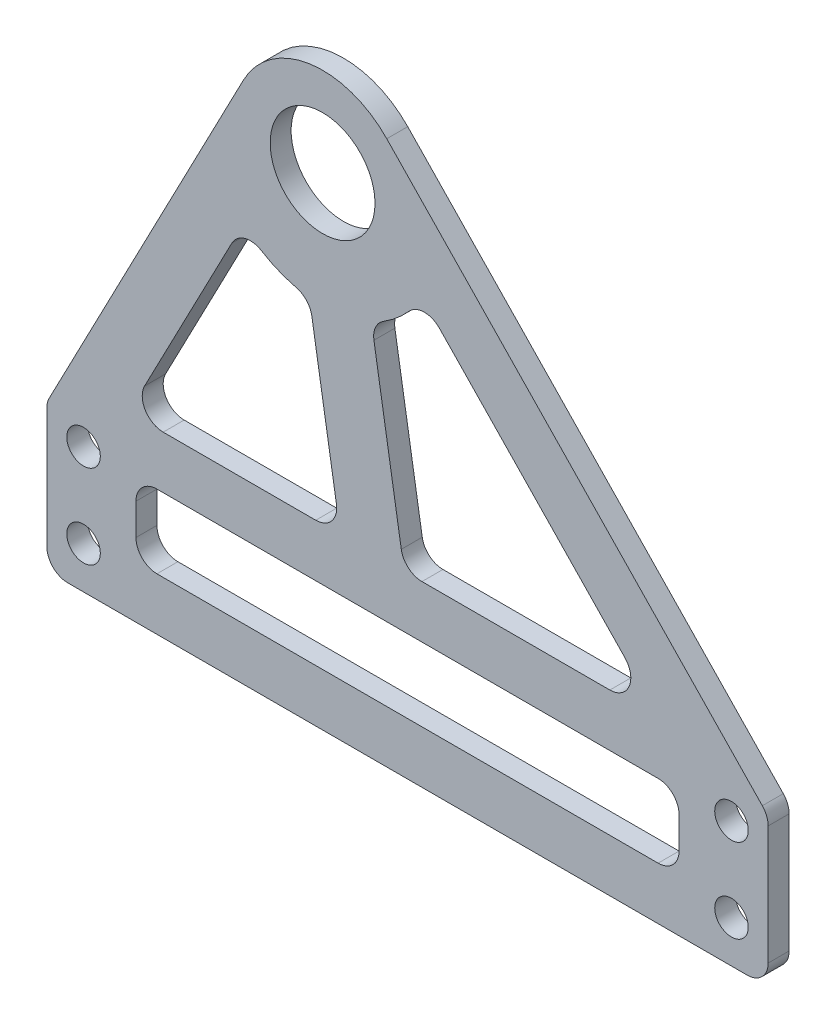
SolidWorks part; units mm, degrees
material "Thornel Mat VMA"
ref_plane "前视基准面" through (0, 0, 0) normal (0, 0, 1) x (1, 0, 0)
ref_plane "上视基准面" through (0, 0, 0) normal (0, 1, 0) x (1, 0, 0)
ref_plane "右视基准面" through (0, 0, 0) normal (1, 0, 0) x (0, 0, -1)
other "Configuration Table"
sketch "草图1" plane through (0, 0, 0) normal (0, 0, 1) x (1, 0, 0)
  line L0 (-26.8, 16.8667) -> (-26.8, -34) construction
  line L1 (43, 15.0741) -> (43, -34) construction
  line L2 (-26.8, -34) -> (43, -34) construction
  line L3 (-22.8, -34) -> (-22.8, -42) construction
  line L4 (8.1, -34) -> (8.1, 15.0741) construction
  line L5 (-26.3, -32.0608) -> (-26.3, -46)
  line L6 (-7.5372, 3.9294) -> (-26.3, -32.0608)
  line L7 (-26.3, -46) -> (42.5, -46)
  line L8 (42.5, -46) -> (42.5, -31.8677)
  line L9 (42.5, -31.8677) -> (6.1217, 5.897)
  circle A0 centre (0, 0) radius 5
  circle A1 centre (-22.8, -34) radius 1.6
  circle A2 centre (-22.8, -42) radius 1.6
  circle A3 centre (39, -42) radius 1.6
  circle A4 centre (39, -34) radius 1.6
  arc A5 (6.1217, 5.897) -> (-7.5372, 3.9294) centre (0, 0) ccw
  dimension "D3" = 10
  dimension "D5" = 3.2
  dimension "D6" = 3.2
  dimension "D10" = 17
  dimension "D1" = 26.8
  dimension "D2" = 43
  dimension "D4" = 34
  dimension "D7" = 8
  dimension "D8" = 4
  dimension "D9" = 0.5
  dimension "D11" = 4
  dimension "D12" = 0.5
  dimension "D13" = 4
  dimension "D14" = 4
extrude "凸台-拉伸1" add sketch "草图1" along normal blind 2
sketch "草图2" plane through (0, 0, 2) normal (0, 0, 1) x (1, 0, 0)
  line L0 (-22.8, -34) -> (-25.3, -34) construction
  line L1 (-25.3, -34) -> (-25.3, -18) construction
  line L2 (-25.3, -17.75) -> (15.7, -17.75) construction
  line L3 (-26.3, -32.0608) -> (-28.2703, -18.1713)
  line L4 (-6.0422, 5.9785) -> (-27.4325, -15.64)
  line L5 (-26.3, -32.0608) -> (-7.5372, 3.9294)
  circle A0 centre (-25.3, -18) radius 2.75 construction
  circle A1 centre (-25.3, -17.75) radius 2.5 construction
  circle A2 centre (-25.3, -17.75) radius 1.6
  circle A3 centre (15.7, -17.75) radius 1.6 construction
  arc A4 (-27.4325, -15.64) -> (-28.2703, -18.1713) centre (-25.3, -17.75) ccw
  arc A5 (6.1217, 5.897) -> (-7.5372, 3.9294) centre (0, 0) ccw construction
  arc A6 (-6.0422, 5.9785) -> (-7.5372, 3.9294) centre (0, 0) ccw
  dimension "D3" = 5.5
  dimension "D4" = 5
  dimension "D5" = 3.2
  dimension "D7" = 3.2
  dimension "D8" = 6
  dimension "D1" = 2.5
  dimension "D2" = 16
  dimension "D6" = 41
extrude "凸台-拉伸2" [suppressed] add sketch "草图2" against normal up to surface (3 mm away)
sketch "草图3" plane through (0, 0, 2) normal (0, 0, 1) x (1, 0, 0)
  circle A0 centre (15.7, -17.75) radius 1.6
  dimension "D1" = 3.2
extrude "切除-拉伸1" [suppressed] cut sketch "草图3" against normal up to surface (3 mm away)
sketch "草图4" [suppressed] plane through (0, 0, 3) normal (0, 0, 1) x (1, 0, 0)
  line L0 (0, 0) -> (-20.5, -17.75) construction
  line L1 (-20.5, -17.75) -> (-18, -34) construction
  line L2 (-18, -34) -> (39, -34) construction
  line L3 (39, -34) -> (20.5, -17.75) construction
  line L4 (20.5, -17.75) -> (0, 0) construction
  line L5 (0, 0) -> (10.5, -34) construction
  line L6 (-14.2121, -31) -> (-16.0014, -19.37)
  line L7 (-16.0014, -19.37) -> (-6.6873, -8.0951)
  line L8 (-14.2121, -31) -> (5.9104, -31)
  line L9 (5.9104, -31) -> (-0.4231, -10.4915)
  line L10 (13.2366, -31) -> (31.2197, -31)
  line L11 (31.2197, -31) -> (20.5364, -21.7498)
  line L12 (13.2366, -31) -> (6.6729, -9.7461)
  line L13 (16.5361, -18.2861) -> (6.6729, -9.7461)
  line L14 (-5.7822, 4.7766) -> (-22.8129, -15.8393) construction
  arc A2 (16.5361, -18.2861) -> (20.5364, -21.7498) centre (20.5, -17.75) ccw
  arc A3 (-6.6873, -8.0951) -> (-0.4231, -10.4915) centre (0, 0) ccw
  dimension "D1" = 10.5
  dimension "D8" = 8
  dimension "D2" = 7.5
  dimension "D3" = 4.2
  dimension "D4" = 3
  dimension "D5" = 3.5
  dimension "D6" = 3.5
  dimension "D7" = 3
extrude "切除-拉伸2" [suppressed] cut sketch "草图4" against normal through all
fillet "圆角1" [suppressed] radius 3
fillet "圆角2" [suppressed] radius 1
fillet "圆角3" [suppressed] radius 2
sketch "草图5" [suppressed] plane through (0, 0, 3) normal (0, 0, 1) x (1, 0, 0)
  line L0 (-18, -34) -> (-18, -42) construction
  line L1 (-13, -36) -> (34, -36)
  line L2 (-13, -36) -> (-13, -41.5)
  line L3 (-13, -41.5) -> (34, -41.5)
  line L4 (34, -36) -> (34, -41.5)
  line L5 (-18, -42) -> (39, -42) construction
  line L6 (-11.6384, -31) -> (1.8442, -31) construction
  dimension "D1" = 5
  dimension "D2" = 5
  dimension "D3" = 0.5
  dimension "D4" = 5
extrude "切除-拉伸3" [suppressed] cut sketch "草图5" against normal through all
fillet "圆角4" [suppressed] radius 2
sketch "草图6" plane through (0, 0, 2) normal (0, 0, 1) x (1, 0, 0)
  line L0 (-7.5525, -7.9975) -> (-18.5018, -29)
  line L1 (-18.5018, -29) -> (1.7, -29)
  line L2 (1.7, -29) -> (-1.2537, -10.9283)
  line L3 (4.6678, -9.9605) -> (7.7796, -29)
  line L4 (7.7796, -29) -> (32.1008, -29)
  line L5 (32.1008, -29) -> (9.5027, -5.5406)
  line L6 (42.5, -31.8677) -> (6.1217, 5.897) construction
  line L7 (-22.8, -34) -> (39, -34) construction
  line L8 (-7.5372, 3.9294) -> (-26.3, -32.0608) construction
  line L9 (-26.3, -46) -> (42.5, -46) construction
  line L10 (-17.8, -34) -> (34, -34)
  line L11 (-17.8, -34) -> (-17.8, -41)
  line L12 (-17.8, -41) -> (34, -41)
  line L13 (34, -34) -> (34, -41)
  arc A0 (-7.5525, -7.9975) -> (-1.2537, -10.9283) centre (0, 0) ccw
  arc A1 (4.6678, -9.9605) -> (9.5027, -5.5406) centre (0, 0) ccw
  dimension "D1" = 22
  dimension "D2" = 5
  dimension "D3" = 6
  dimension "D4" = 5.5
  dimension "D5" = 5.5
  dimension "D6" = 3
  dimension "D7" = 24.5
  dimension "D8" = 5
  dimension "D9" = 5
  dimension "D10" = 5
  dimension "D11" = 5
extrude "切除-拉伸4" cut sketch "草图6" against normal through all
fillet "圆角5" radius 2 12 edges at (1.7, -29, 1) (-18.5018, -29, 1) (-7.5525, -7.9975, 1) (-1.2537, -10.9283, 1) (32.1008, -29, 1) (7.7796, -29, 1) (4.6678, -9.9605, 1) (9.5027, -5.5406, 1) (34, -34, 1) (34, -41, 1) (-17.8, -41, 1) (-17.8, -34, 1)
fillet "圆角6" radius 2 4 edges at (42.5, -31.8677, 1) (42.5, -46, 1) (-26.3, -32.0608, 1) (-26.3, -46, 1)
